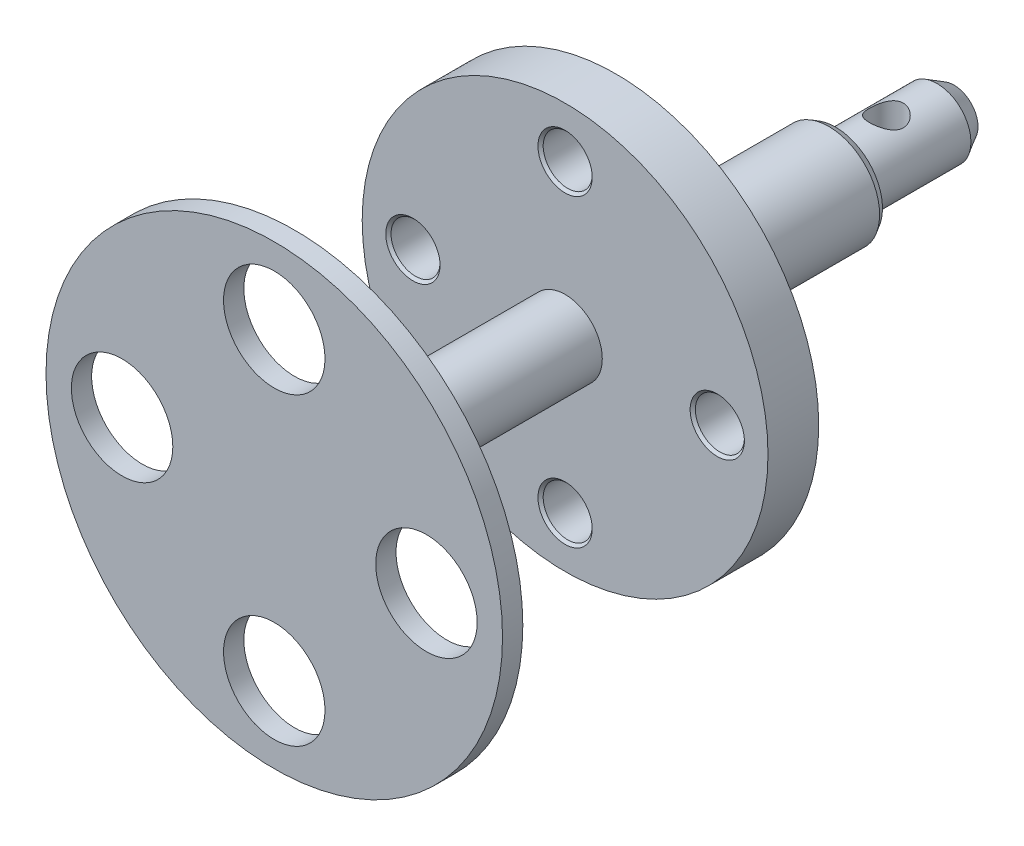
from build123d import *

# Parameters (mm, degrees)
SKETCH1_R               = 52.5
SKETCH1_R_2             = 3.5
BOSS_EXTRUDE1_DEPTH     = 14
SKETCH2_R               = 10
BOSS_EXTRUDE2_DEPTH     = 100
SKETCH3_R               = 60
BOSS_EXTRUDE3_DEPTH     = 15
CIRPATTERN1_COUNT       = 4
SKETCH6_R               = 67.698937757
CUT_EXTRUDE1_DEPTH      = 14
CHAMFER1_SIZE           = 5
CHAMFER1_SIZE2          = 2.886751346
CUT_EXTRUDE2_DEPTH      = 155.405310789
CUT_EXTRUDE2_DEPTH_BACK = 155.405310789
SKETCH7_R               = 5
SKETCH8_R               = 15
BOSS_EXTRUDE4_DEPTH     = 65
CHAMFER2_SIZE           = 2
CHAMFER2_SIZE2          = 1.154700538
SKETCH9_R               = 11
BOSS_EXTRUDE5_DEPTH     = 80
SKETCH10_R              = 67.5
SKETCH10_R_2            = 15
BOSS_EXTRUDE6_DEPTH     = 6


with BuildPart() as part:
    # Sketch1 → Boss-Extrude1 (new body)
    with BuildSketch(Plane.XY):
        Circle(SKETCH1_R)
        with Locations((0, 45)):
            Circle(SKETCH1_R_2, mode=Mode.SUBTRACT)
        with Locations((38.97114317, 22.5)):
            Circle(SKETCH1_R_2, mode=Mode.SUBTRACT)
        with Locations((38.97114317, -22.5)):
            Circle(SKETCH1_R_2, mode=Mode.SUBTRACT)
        with Locations((0, -45)):
            Circle(SKETCH1_R_2, mode=Mode.SUBTRACT)
        with Locations((-38.97114317, -22.5)):
            Circle(SKETCH1_R_2, mode=Mode.SUBTRACT)
        with Locations((-38.97114317, 22.5)):
            Circle(SKETCH1_R_2, mode=Mode.SUBTRACT)
    extrude(amount=BOSS_EXTRUDE1_DEPTH)

    # Sketch2 → Boss-Extrude2 (add)
    with BuildSketch(Plane.XY.offset(14)):
        Circle(SKETCH2_R)
    extrude(amount=BOSS_EXTRUDE2_DEPTH)

    # Sketch3 → Boss-Extrude3 (add)
    with BuildSketch(Plane.XY.offset(114)):
        Circle(SKETCH3_R)
    extrude(amount=BOSS_EXTRUDE3_DEPTH)

    # Sketch5 → M16x1.5 Tapped Hole1 (revolve, cut)
    with BuildSketch(Plane(origin=(0, 45, 129), x_dir=(0, -1, 0), z_dir=(1, 0, 0))):
        Polygon((0, 0), (0, 40.856239488), (7.25, 36.5), (7.25, 0.775), (8.025, 0), align=None)
    m16x1_5_tapped_hole1 = revolve(axis=Axis((0, 45, 135.35), (0, 0, -1)), mode=Mode.SUBTRACT)

    # CirPattern1: M16x1.5 Tapped Hole1 ×4 about axis
    cirpattern1_axis = Axis((0, 0, 0), (0, 0, 1))
    for i in range(1, CIRPATTERN1_COUNT):
        add(m16x1_5_tapped_hole1.rotate(cirpattern1_axis, i * 360 / CIRPATTERN1_COUNT), mode=Mode.SUBTRACT)

    # Sketch6 → Cut-Extrude1 (cut)
    with BuildSketch(Plane(origin=(0, 0, 0), x_dir=(-1, 0, 0), z_dir=(0, 0, -1))):
        Circle(SKETCH6_R)
    extrude(amount=-CUT_EXTRUDE1_DEPTH, mode=Mode.SUBTRACT)

    # Chamfer1
    chamfer1_edges = [part.edges().sort_by_distance(p)[0] for p in [
        (-10, 0, 14),
    ]]
    chamfer1_side = [part.faces().sort_by_distance(p)[0] for p in [
        (-10, 0, 64),
    ]]
    chamfer(chamfer1_edges, length=CHAMFER1_SIZE, length2=CHAMFER1_SIZE2, reference=chamfer1_side[0])

    # Sketch7 → Cut-Extrude2 (cut, two sides: drawn at the far end of the back side and taken through both)
    with BuildSketch(Plane(origin=(0, 0, 0), x_dir=(1, 0, 0), z_dir=(0, 1, 0)).offset(-CUT_EXTRUDE2_DEPTH_BACK)):
        with Locations(Location((0, -34, 0), (0, 0, 270))):
            Circle(SKETCH7_R)
    extrude(amount=CUT_EXTRUDE2_DEPTH + CUT_EXTRUDE2_DEPTH_BACK, mode=Mode.SUBTRACT)

    # Sketch8 → Boss-Extrude4 (add)
    with BuildSketch(Plane(origin=(0, 0, 114), x_dir=(-1, 0, 0), z_dir=(0, 0, -1))):
        with Locations(Location((0, 0, 0), (0, 0, 180))):
            Circle(SKETCH8_R)
    extrude(amount=BOSS_EXTRUDE4_DEPTH)

    # Chamfer2
    chamfer2_edges = [part.edges().sort_by_distance(p)[0] for p in [
        (-15, 0, 49),
    ]]
    chamfer2_side = [part.faces().sort_by_distance(p)[0] for p in [
        (-15, 0, 81.5),
    ]]
    chamfer(chamfer2_edges, length=CHAMFER2_SIZE, length2=CHAMFER2_SIZE2, reference=chamfer2_side[0])

    # Sketch9 → Boss-Extrude5 (add)
    with BuildSketch(Plane.XY.offset(129)):
        Circle(SKETCH9_R)
    extrude(amount=BOSS_EXTRUDE5_DEPTH)

    # Sketch10 → Boss-Extrude6 (add)
    with BuildSketch(Plane.XY.offset(209)):
        Circle(SKETCH10_R)
        with Locations((0, 45)):
            Circle(SKETCH10_R_2, mode=Mode.SUBTRACT)
        with Locations((45, 0)):
            Circle(SKETCH10_R_2, mode=Mode.SUBTRACT)
        with Locations((0, -45)):
            Circle(SKETCH10_R_2, mode=Mode.SUBTRACT)
        with Locations((-45, 0)):
            Circle(SKETCH10_R_2, mode=Mode.SUBTRACT)
    extrude(amount=BOSS_EXTRUDE6_DEPTH)


solid = part.part
